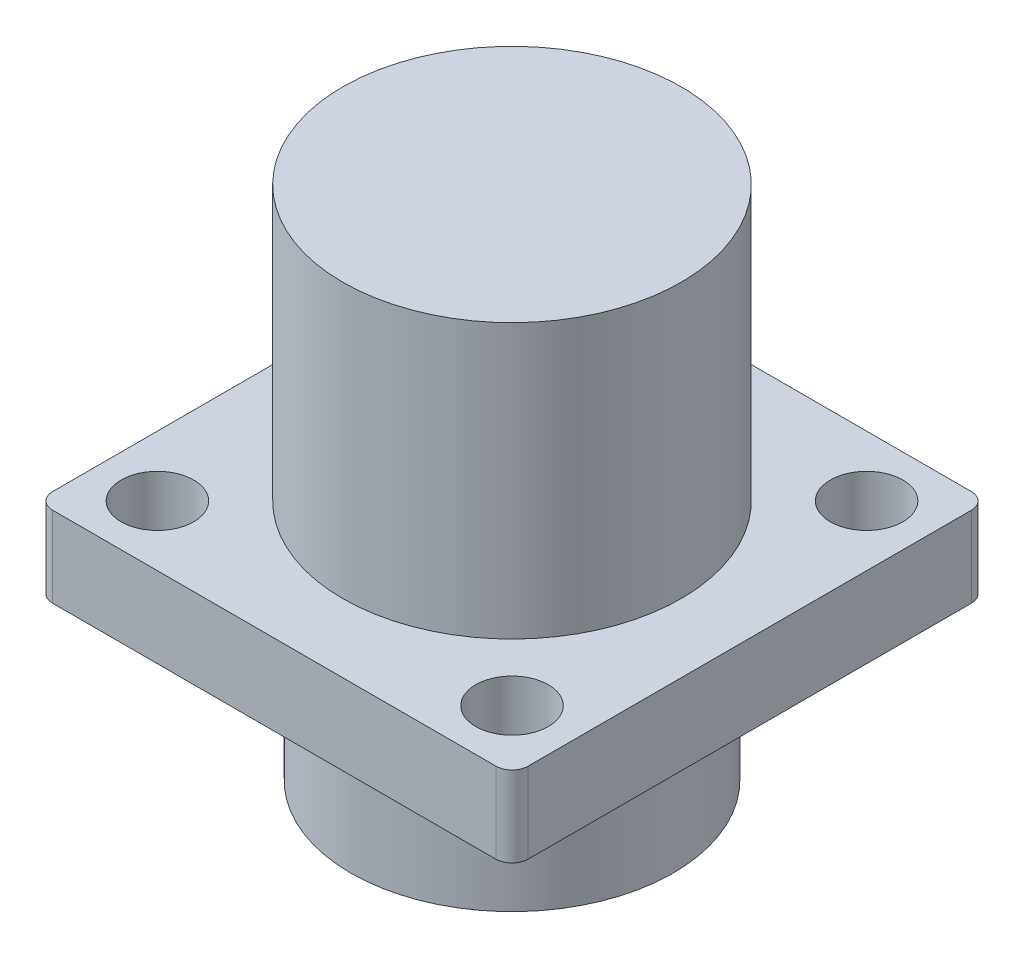
SolidWorks part; units mm, degrees
ref_plane "前视基准面" through (0, 0, 0) normal (0, 0, 1) x (1, 0, 0)
ref_plane "上视基准面" through (0, 0, 0) normal (0, 1, 0) x (1, 0, 0)
ref_plane "右视基准面" through (0, 0, 0) normal (1, 0, 0) x (0, 0, -1)
sketch "草图1" plane through (0, 0, 0) normal (0, 1, 0) x (1, 0, 0)
  circle A0 centre (0, 0) radius 10
  dimension "D1" = 20
extrude "凸台-拉伸1" add sketch "草图1" along normal blind 10
sketch "草图2" plane through (0, 10, 0) normal (0, 1, 0) x (1, 0, 0)
  line L1 (-14.75, 14.75) -> (14.75, 14.75)
  line L2 (-14.75, 14.75) -> (-14.75, -14.75)
  line L3 (-14.75, -14.75) -> (14.75, -14.75)
  line L4 (14.75, 14.75) -> (14.75, -14.75)
  line L5 (-14.75, 14.75) -> (14.75, -14.75) construction
  line L6 (-14.75, -14.75) -> (14.75, 14.75) construction
  point P0 (0, 0)
  dimension "D1" = 29.5
extrude "凸台-拉伸2" add sketch "草图2" along normal blind 5
sketch "草图3" plane through (0, 15, 0) normal (0, 1, 0) x (1, 0, 0)
  circle A0 centre (0, 0) radius 10.5
  dimension "D1" = 21
extrude "凸台-拉伸3" add sketch "草图3" along normal blind 17
sketch "草图4" plane through (0, 15, 0) normal (0, 1, 0) x (1, 0, 0)
  line L1 (-11, 11) -> (11, 11) construction
  line L2 (-11, 11) -> (-11, -11) construction
  line L3 (-11, -11) -> (11, -11) construction
  line L4 (11, 11) -> (11, -11) construction
  line L5 (-11, 11) -> (11, -11) construction
  line L6 (-11, -11) -> (11, 11) construction
  circle A0 centre (11, 11) radius 2.25
  circle A1 centre (-11, 11) radius 2.25
  circle A2 centre (-11, -11) radius 2.25
  circle A3 centre (11, -11) radius 2.25
  point P0 (0, 0)
  dimension "D2" = 4.5
  dimension "D1" = 22
extrude "切除-拉伸1" cut sketch "草图4" against normal blind 17
fillet "圆角1" radius 1 4 edges at (-14.75, 12.5, -14.75) (14.75, 12.5, -14.75) (14.75, 12.5, 14.75) (-14.75, 12.5, 14.75)
